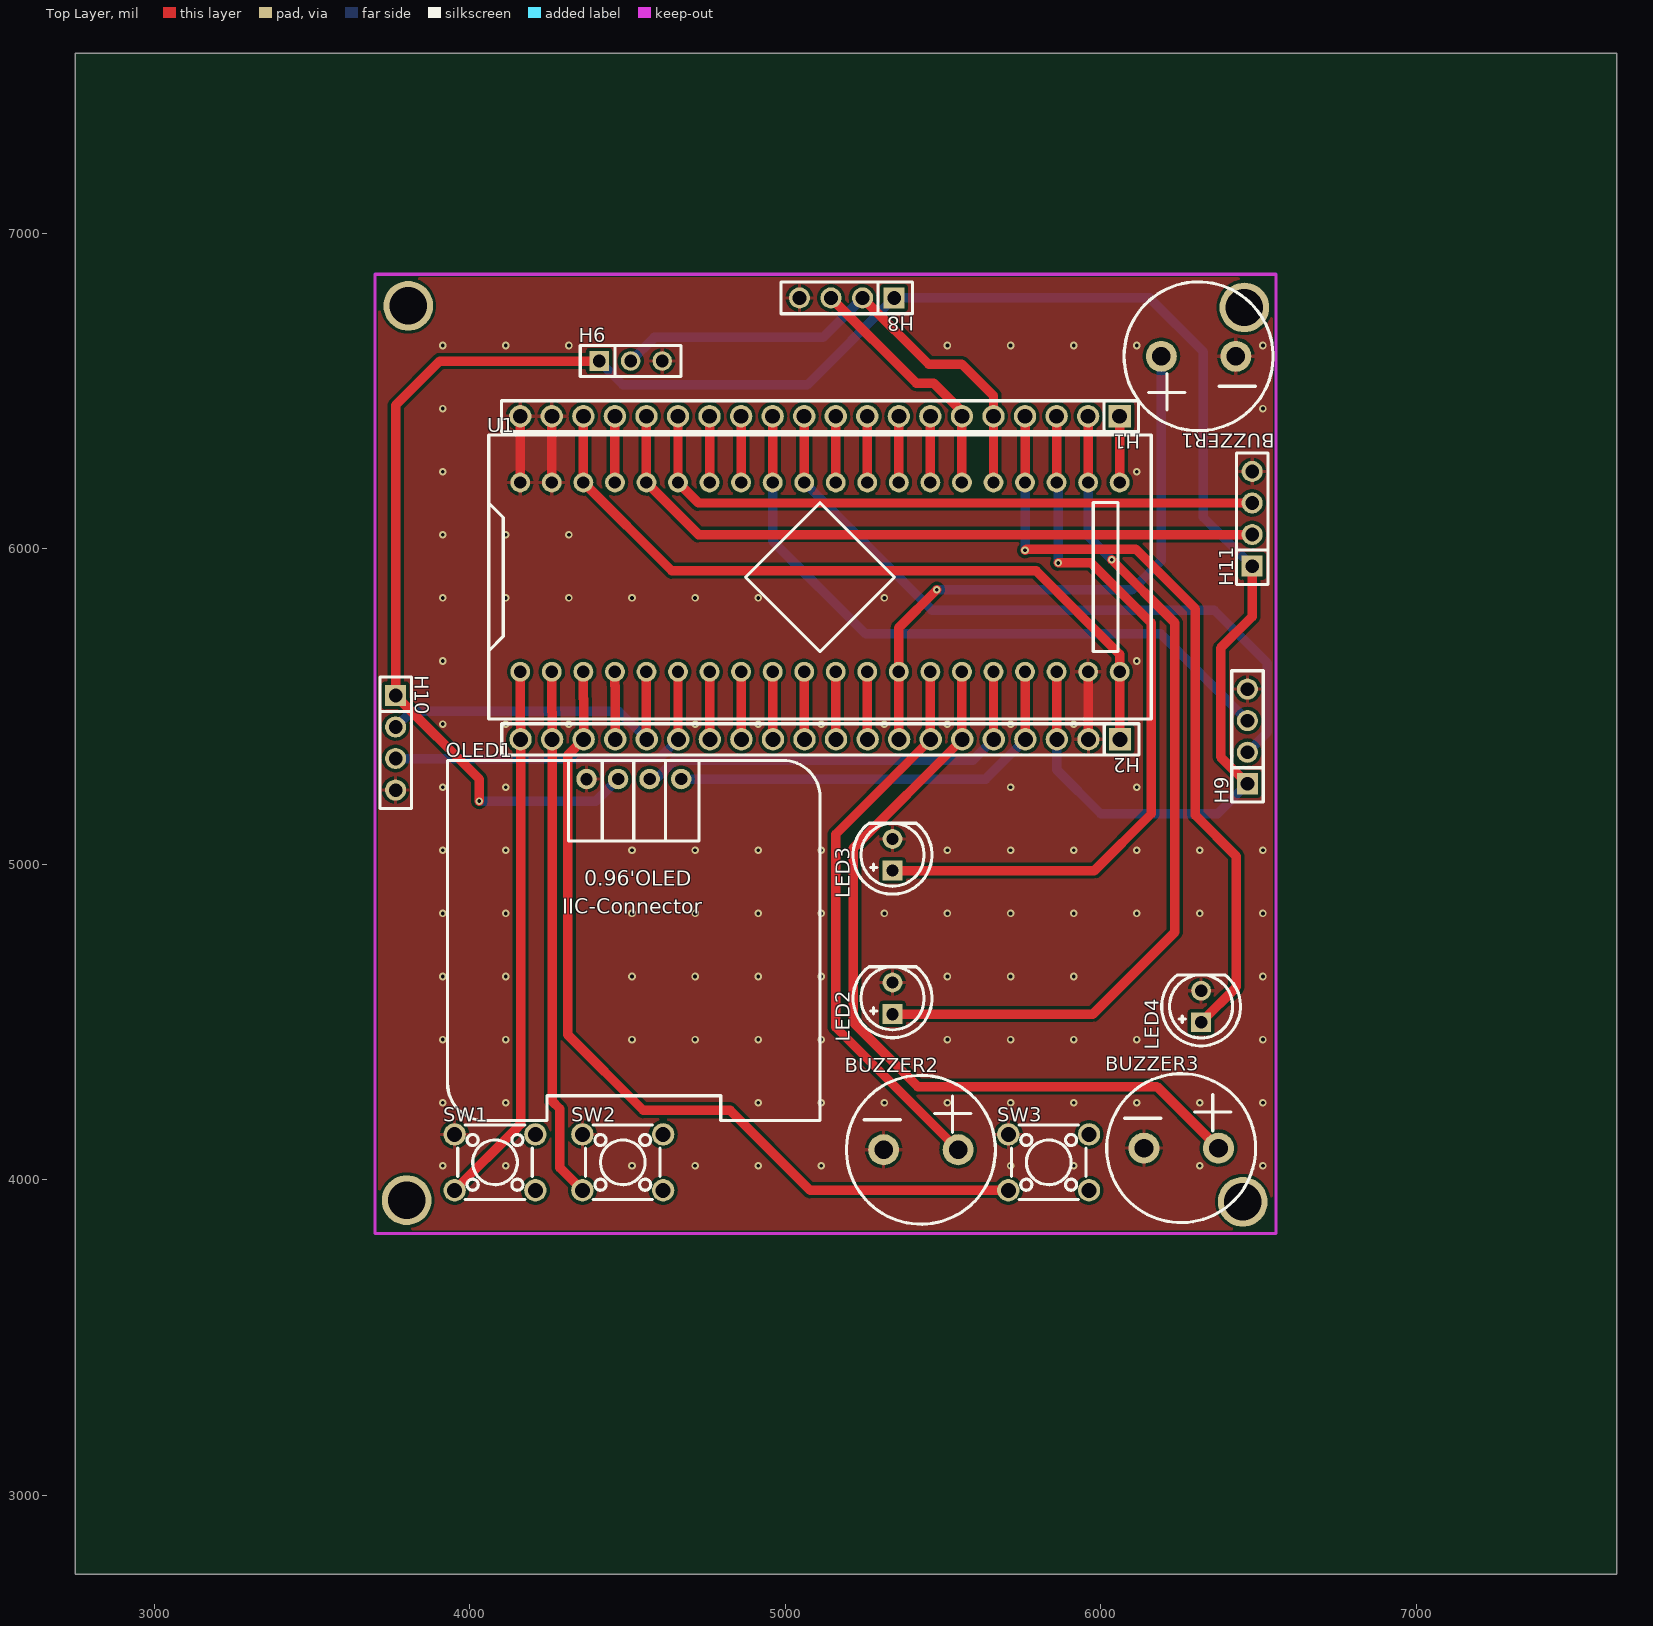
[diagram p0: Top Layer view]
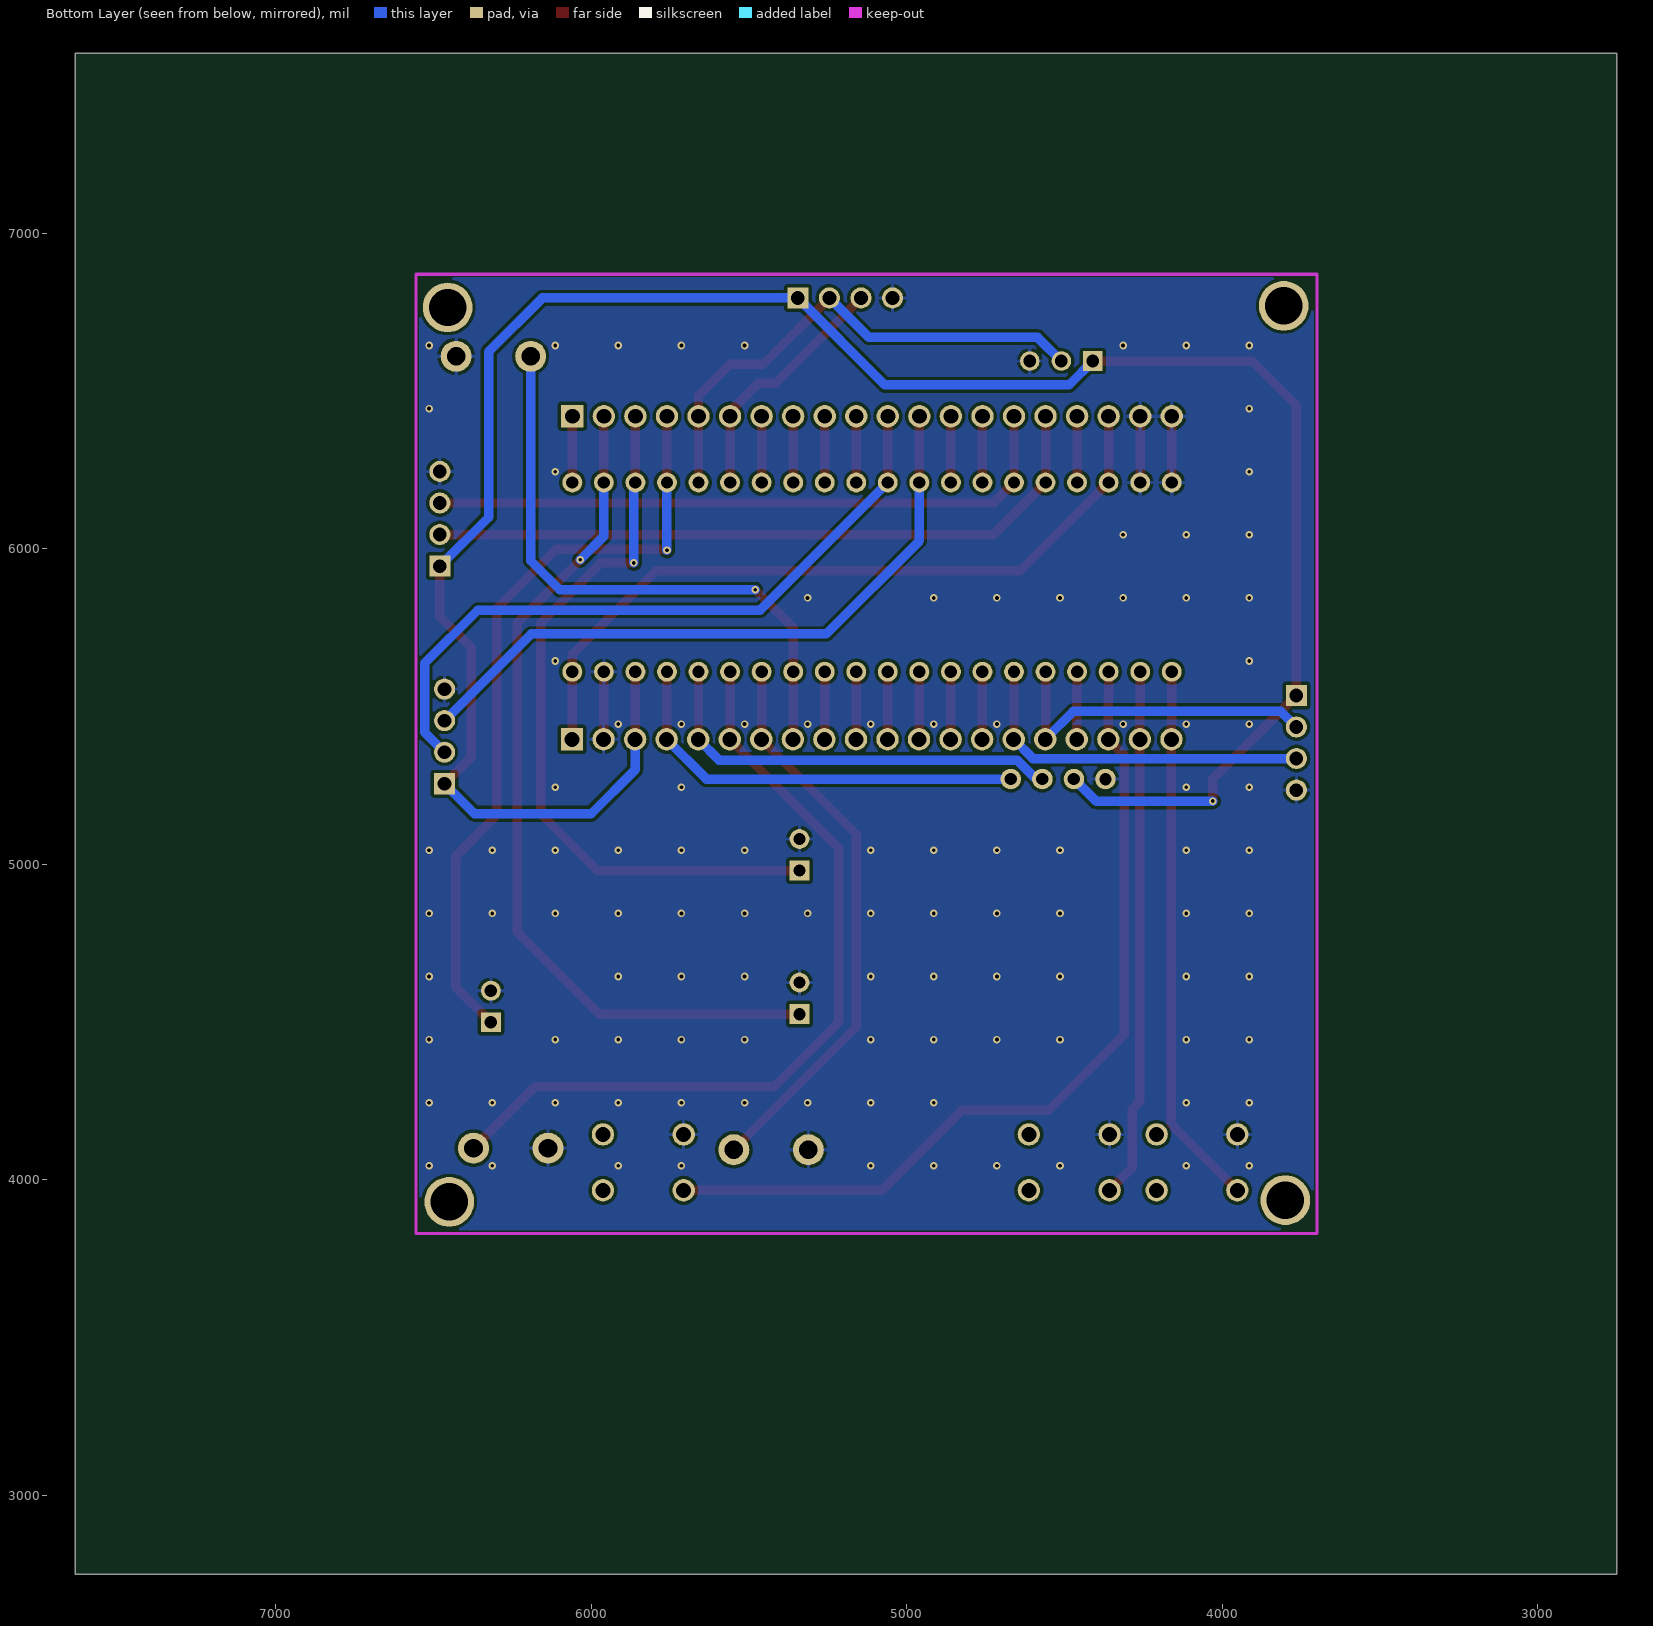
[diagram p1: Bottom Layer view, seen from below]
# Altium PCB MISC51974.pcbdoc
Units mil, origin at the board's own origin, x right, y up, seen from the top; angles counter-clockwise.
Board outline 4885 x 4820 mil, 2 copper layers (Top Layer, Bottom Layer), stack 62.206 mil thick; 18 components, 37 nets, 131 pads, 110 vias.

## Layer stack, top to bottom
Top Solder Mask Layer: solder mask 0.394, Dk 3.3
Top Layer: signal copper 1.379
Dielectric1: surface 59.449, FR4, Dk 4.5
Bottom Layer: signal copper 1.378
Bottom Solder Mask Layer: solder mask 0.394, Dk 3.3

## Board outline
7635,2750 2750,2750 2750,7570 7635,7570

## Design rules (kind name [scope] priority, off if disabled: settings)
BoardOutlineClearance copperThickness2oz_1 [All] p2 off: genericclearance=7.99 ignorepadtopadclearanceinfootprint=FALSE except(0: Arc-SplitContinuation Track-SplitContinuation SMDPad-SplitContinuation THPad-SplitContinuation Via-SplitContinuation Fill-SplitContinuation Region-SplitContinuation Poly-SplitContinuation Text-SplitContinuation Hole-SplitContinuation; 5.98: Arc-CutoutEdge Track-CutoutEdge SMDPad-CutoutEdge THPad-CutoutEdge Via-CutoutEdge Text-CutoutEdge; 6.89: Hole-OutlineEdge Hole-CutoutEdge; 10: Poly-OutlineEdge Poly-CutoutEdge; 11.81: Arc-OutlineEdge Track-OutlineEdge SMDPad-OutlineEdge THPad-OutlineEdge Via-OutlineEdge Fill-OutlineEdge Region-OutlineEdge Text-OutlineEdge Fill-CutoutEdge Region-CutoutEdge)
BoardOutlineClearance Plane_innerPlane_1 [All] p4 off: genericclearance=4.02 ignorepadtopadclearanceinfootprint=FALSE except(0: Arc-SplitContinuation Track-SplitContinuation SMDPad-SplitContinuation THPad-SplitContinuation Via-SplitContinuation Fill-SplitContinuation Region-SplitContinuation Poly-SplitContinuation Text-SplitContinuation Hole-SplitContinuation; 5.98: Arc-CutoutEdge Track-CutoutEdge SMDPad-CutoutEdge THPad-CutoutEdge Via-CutoutEdge Text-CutoutEdge; 6.89: Hole-OutlineEdge Hole-CutoutEdge; 10: Poly-OutlineEdge Poly-CutoutEdge; 11.81: Arc-OutlineEdge Track-OutlineEdge SMDPad-OutlineEdge THPad-OutlineEdge Via-OutlineEdge Fill-OutlineEdge Region-OutlineEdge Text-OutlineEdge Fill-CutoutEdge Region-CutoutEdge)
BoardOutlineClearance Copper_copperRegion_1 [All] p6 off: genericclearance=4.02 ignorepadtopadclearanceinfootprint=FALSE except(0: Arc-SplitContinuation Track-SplitContinuation SMDPad-SplitContinuation THPad-SplitContinuation Via-SplitContinuation Fill-SplitContinuation Region-SplitContinuation Poly-SplitContinuation Text-SplitContinuation Hole-SplitContinuation; 5.98: Arc-CutoutEdge Track-CutoutEdge SMDPad-CutoutEdge THPad-CutoutEdge Via-CutoutEdge Text-CutoutEdge; 6.89: Hole-OutlineEdge Hole-CutoutEdge; 10: Poly-OutlineEdge Poly-CutoutEdge; 11.81: Arc-OutlineEdge Track-OutlineEdge SMDPad-OutlineEdge THPad-OutlineEdge Via-OutlineEdge Fill-OutlineEdge Region-OutlineEdge Text-OutlineEdge Fill-CutoutEdge Region-CutoutEdge)
BoardOutlineClearance copperThickness1oz_1 [All] p8: genericclearance=4.02 ignorepadtopadclearanceinfootprint=FALSE except(0: Arc-SplitContinuation Track-SplitContinuation SMDPad-SplitContinuation THPad-SplitContinuation Via-SplitContinuation Fill-SplitContinuation Region-SplitContinuation Poly-SplitContinuation Text-SplitContinuation Hole-SplitContinuation; 5.98: Arc-CutoutEdge Track-CutoutEdge SMDPad-CutoutEdge THPad-CutoutEdge Via-CutoutEdge Text-CutoutEdge; 6.89: Hole-OutlineEdge Hole-CutoutEdge; 10: Poly-OutlineEdge Poly-CutoutEdge; 11.81: Arc-OutlineEdge Track-OutlineEdge SMDPad-OutlineEdge THPad-OutlineEdge Via-OutlineEdge Fill-OutlineEdge Region-OutlineEdge Text-OutlineEdge Fill-CutoutEdge Region-CutoutEdge)
Clearance copperThickness2oz [All] p1 off: gap=7.99 ignorepadtopadclearanceinfootprint=FALSE except(5.98: SMDPad-Track SMDPad-SMDPad THPad-Track SMDPad-THPad THPad-THPad Track-Via SMDPad-Via THPad-Via Via-Via Fill-SMDPad Region-SMDPad Fill-THPad Region-THPad Fill-Via Region-Via Fill-Fill Fill-Region Region-Region Arc-Track Arc-SMDPad Arc-THPad Arc-Via Fill-Arc Region-Arc Arc-Arc Text-Track SMDPad-Text Text-THPad Text-Via Fill-Text Region-Text Arc-Text Text-Text; 6.89: Hole-Track Hole-SMDPad Hole-THPad Hole-Via Fill-Hole Region-Hole Hole-Arc Hole-Text; 10: Poly-Track Poly-SMDPad Poly-THPad Poly-Via Poly-Fill Poly-Region Poly-Poly Poly-Arc Poly-Text Poly-Hole; 11.81: Fill-Track Region-Track)
Clearance Plane_innerPlane [All] p3 off: gap=4.02 ignorepadtopadclearanceinfootprint=FALSE except(5.98: SMDPad-Track SMDPad-SMDPad THPad-Track SMDPad-THPad THPad-THPad Track-Via SMDPad-Via THPad-Via Via-Via Fill-SMDPad Region-SMDPad Fill-THPad Region-THPad Fill-Via Region-Via Fill-Fill Fill-Region Region-Region Arc-Track Arc-SMDPad Arc-THPad Arc-Via Fill-Arc Region-Arc Arc-Arc Text-Track SMDPad-Text Text-THPad Text-Via Fill-Text Region-Text Arc-Text Text-Text; 6.89: Hole-Track Hole-SMDPad Hole-THPad Hole-Via Fill-Hole Region-Hole Hole-Arc Hole-Text; 10: Poly-Track Poly-SMDPad Poly-THPad Poly-Via Poly-Fill Poly-Region Poly-Poly Poly-Arc Poly-Text Poly-Hole; 11.81: Fill-Track Region-Track)
Clearance Copper_copperRegion [All] p5 off: gap=4.02 ignorepadtopadclearanceinfootprint=FALSE except(5.98: SMDPad-Track SMDPad-SMDPad THPad-Track SMDPad-THPad THPad-THPad Track-Via SMDPad-Via THPad-Via Via-Via Fill-SMDPad Region-SMDPad Fill-THPad Region-THPad Fill-Via Region-Via Fill-Fill Fill-Region Region-Region Arc-Track Arc-SMDPad Arc-THPad Arc-Via Fill-Arc Region-Arc Arc-Arc Text-Track SMDPad-Text Text-THPad Text-Via Fill-Text Region-Text Arc-Text Text-Text; 6.89: Hole-Track Hole-SMDPad Hole-THPad Hole-Via Fill-Hole Region-Hole Hole-Arc Hole-Text; 10: Poly-Track Poly-SMDPad Poly-THPad Poly-Via Poly-Fill Poly-Region Poly-Poly Poly-Arc Poly-Text Poly-Hole; 11.81: Fill-Track Region-Track)
Clearance copperThickness1oz [All] p7: gap=4.02 ignorepadtopadclearanceinfootprint=FALSE except(5.98: SMDPad-Track SMDPad-SMDPad THPad-Track SMDPad-THPad THPad-THPad Track-Via SMDPad-Via THPad-Via Via-Via Fill-SMDPad Region-SMDPad Fill-THPad Region-THPad Fill-Via Region-Via Fill-Fill Fill-Region Region-Region Arc-Track Arc-SMDPad Arc-THPad Arc-Via Fill-Arc Region-Arc Arc-Arc Text-Track SMDPad-Text Text-THPad Text-Via Fill-Text Region-Text Arc-Text Text-Text; 6.89: Hole-Track Hole-SMDPad Hole-THPad Hole-Via Fill-Hole Region-Hole Hole-Arc Hole-Text; 10: Poly-Track Poly-SMDPad Poly-THPad Poly-Via Poly-Fill Poly-Region Poly-Poly Poly-Arc Poly-Text Poly-Hole; 11.81: Fill-Track Region-Track)
DiffPairsRouting differentialPair [All] p1: maxlimit=6 minlimit=6 mostfreqgap=6 toplayer_minwidth=5 toplayer_prefwidth=10 toplayer_maxwidth=100 toplayer_mingap=6 toplayer_prefgap=6 toplayer_maxgap=6 bottomlayer_minwidth=5 bottomlayer_prefwidth=10 bottomlayer_maxwidth=100 bottomlayer_mingap=6 bottomlayer_prefgap=6 bottomlayer_maxgap=6 maxuncoupledlength=10
HoleToHoleClearance otherClearance [All] p1: gap=11.81 allowstackedmicrovias=TRUE
Length netLength [All] p1: minlimit=0 maxlimit=0
PasteMaskExpansion pasteMaskExpansion [All] p1: expansion=0
PlaneConnect innerPlane [All] p1: planeconnectstyle=Relief reliefexpansion=20 reliefentries=4 reliefconductorwidth=10 reliefairgap=10
PolygonConnect copperRegion [All] p1: connectstyle=Relief reliefconductorwidth=10 reliefentries=4 polygonreliefangle="90 Angle" airgapwidth=10 via.connectstyle=Relief via.reliefconductorwidth=10 via.reliefentries=4 via.polygonreliefangle="90 Angle" via.airgapwidth=10
RoutingVias viaSize [All] p1: holewidth=12.01 width=24.02 viastyle="Through Hole" minholewidth=11.81 minwidth=19.68 maxholewidth=248.03 maxwidth=393.7
SolderMaskExpansion solderMaskExpansion [IsVia] p1: expansion=-1000 istentingtop=TRUE
SolderMaskExpansion solderMaskExpansion [All] p2: expansion=2.01 istentingtop=FALSE
Width copperThickness2oz_2 [All] p1 off: maxlimit=100 minlimit=8 preferedwidth=10
Width copperThickness1oz_2 [All] p2: maxlimit=100 minlimit=5 preferedwidth=30

## Components (designator, comment, footprint, x,y, rotation, side; value= is the part's Value field where it differs from the comment)
BUZZER1 "buzzer" BUZ-TH_BD12.0-P6.00-D0.9-RD 6310,6610 r180 top
BUZZER2 "buzzer" BUZ-TH_BD12.0-P6.00-D0.9-RD 5430,4095 r0 top
BUZZER3 "buzzer" BUZ-TH_BD12.0-P6.00-D0.9-RD 6255,4100 r0 top
H1 "" HDR-TH_20P-P2.54-V-F 5110,6420 r180 top
H2 "" HDR-TH_20P-P2.54-V-F 5110.96,5395.9 r180 top
H6 "" HDR-TH_3P-P2.54-V-F 4510,6595 r0 top
H8 "" HDR-TH_4P-P2.54-V-F 5195,6795 r180 top
H9 "" HDR-TH_4P-P2.54-V-F 6465,5405 r90 top
H10 "" HDR-TH_4P-P2.54-V-F 3765,5385 r270 top
H11 "" HDR-TH_4P-P2.54-V-F 6480,6095 r90 top
LED2 "" LED-TH_5mm 5340,4575 r90 top
LED3 "" LED-TH_5mm 5340,5030 r90 top
LED4 "" LED-TH_5mm 6318.09,4549.15 r90 top
OLED1 "" 0.96OLED_4P 4520,5270 r0 top
SW1 "" SW-TH_4P-L6.0-W6.0-P4.50-LS6.5 4080,4055 r0 top
SW2 "" SW-TH_4P-L6.0-W6.0-P4.50-LS6.5 4485,4055 r0 top
SW3 "" SW-TH_4P-L6.0-W6.0-P4.50-LS6.5 5835,4055 r0 top
U1 "STM32F103C8T6-Card" CONN-TH_L53.3-W22.9_STM32F103C8T6-CARD 5110,5910 r0 top

## Footprints (in the part's own frame and the unit in brackets; to place one, negate y for a bottom-side part, rotate by r counter-clockwise, add the part's x,y. Pads: shape width x height; smd on the part's side, far side on the other; paste and mask are expansions set on the pad)
0.96OLED_4P [mm]
  round 1.65 hole 1 copper offset 0,0: 1(-3.81,-0.001) 2(-1.27,0.002) 3(1.27,0.002) 4(3.81,0.002)
  silkscreen extent -15,-27.5 15,1.5
BUZ-TH_BD12.0-P6.00-D0.9-RD [mm]
  round 2.5 hole 1.5 paste+0 mask+0.05: 1(-3,0) 2(3,0)
  silkscreen extent -5.99,-5.99 5.99,5.99
CONN-TH_L53.3-W22.9_STM32F103C8T6-CARD [mm]
  round 1.6 hole 1: 1(-24.13,-7.62) 2(-21.59,-7.62) 3(-19.05,-7.62) 4(-16.51,-7.62) 5(-13.97,-7.62) 6(-11.43,-7.62) 7(-8.89,-7.62) 8(-6.35,-7.62) 9(-3.81,-7.62) 10(-1.27,-7.62) 11(1.27,-7.62) 12(3.81,-7.62) 13(6.35,-7.62) 14(8.89,-7.62) 15(11.43,-7.62) 16(13.97,-7.62) 17(16.51,-7.62) 18(19.05,-7.62) 19(21.59,-7.62) 20(24.13,-7.62) 21(24.13,7.62) 22(21.59,7.62) 23(19.05,7.62) 24(16.51,7.62) 25(13.97,7.62) 26(11.43,7.62) 27(8.89,7.62) 28(6.35,7.62) 29(3.81,7.62) 30(1.27,7.62) 31(-1.27,7.62) 32(-3.81,7.62) 33(-6.35,7.62) 34(-8.89,7.62) 35(-11.43,7.62) 36(-13.97,7.62) 37(-16.51,7.62) 38(-19.05,7.62) 39(-21.59,7.62) 40(-24.13,7.62)
  silkscreen extent -26.67,-11.43 26.67,11.43
HDR-TH_3P-P2.54-V-F [mil]
  rect 62x62 hole 40.16: 1(-100,0)
  round 62 hole 40.16: 2(0,0) 3(100,0)
  silkscreen extent -160,-49 160,49
HDR-TH_4P-P2.54-V-F [mm]
  rect 1.7x1.7 hole 1.1: 1(-3.81,0)
  round 1.7 hole 1.1: 2(-1.27,0) 3(1.27,0) 4(3.81,0)
  silkscreen extent -5.29,-1.27 5.29,1.27
HDR-TH_20P-P2.54-V-F [mm]
  rect 1.8x1.8 hole 1.2: 1(-24.13,0)
  round 1.8 hole 1.2: 2(-21.59,0) 3(-19.05,0) 4(-16.51,0) 5(-13.97,0) 6(-11.43,0) 7(-8.89,0) 8(-6.35,0) 9(-3.81,0) 10(-1.27,0) 11(1.27,0) 12(3.81,0) 13(6.35,0) 14(8.89,0) 15(11.43,0) 16(13.97,0) 17(16.51,0) 18(19.05,0) 19(21.59,0) 20(24.13,0)
  silkscreen extent -25.65,-1.25 25.65,1.25
LED-TH_5mm [mm]
  rect 1.6x1.6 hole 1 paste+0 mask+0.051: 1(-1.27,0)
  round 1.6 hole 1 paste+0 mask+0.051: 2(1.27,0)
  silkscreen extent -3.17,-3.17 2.54,3.17
SW-TH_4P-L6.0-W6.0-P4.50-LS6.5 [mm]
  round 1.8 hole 1.2: 1(-3.25,2.25) 2(3.25,2.25) 3(-3.25,-2.25) 4(3.25,-2.25)
  silkscreen extent -3,-3 3,3

## Free pads (board coordinates)
  round 157.48 hole 118.11: 1(3800,3935) 1(3805,6770) 1(6450,3930) 1(6455,6765)

## Via types
v1: diameter 24.02, hole 12, Top Layer to Bottom Layer, 110 vias

## Nets (pads, with @x,y where several pads share a name; then routed paths per layer and width w, separated by ;. In a path a pad name is that pad's centre, name@x,y a point inside that pad or via, vN(x,y) a via of type N, cw(c..) or ccw(c..) an arc to the next point about the centre after c; other vN are vias at no path point)
+5V: H2.3 H6.1 H8.1 H9.1 H10.1 H11.1 OLED1.2 U1.18 | length 7190.3
  Top Layer w30: v1(4030,5200) 4030,5270 H10.1 3765,6455 3905,6595 H6.1 ; U1.18 5860,5396.86 H2.3 ; H9.1 6380,5340 6380,5685 6480,5785 H11.1
  Bottom Layer w30: v1(4030,5200) 4399.95,5200 OLED1.2@4470,5270.05 ; H6.1 4485,6520 5070,6520 H8.1 6155,6795 6325,6625 6325,6100 H11.1 ; H2.3 5860.96,5299.04 6000,5160 6370,5160 H9.1
GND: BUZZER1.1 BUZZER2.1 BUZZER3.1 H1.19 H1.20 H2.2 H6.3 H8.4 H9.4 H10.4 H11.4 LED2.2 LED3.2 LED4.2 OLED1.1 SW1.1 SW2.1 SW3.1 U1.19 U1.39 U1.40 | length 634.5
  Top Layer w30: U1.40 H1.20 ; U1.39 H1.19 ; U1.19 5960,5396.86 H2.2
  other v1: 3914.1,4044.1 4114.1,4044.1 4514.1,4044.1 4714.1,4044.1 4914.1,4044.1 5114.1,4044.1 5714.1,4044.1 5914.1,4044.1 6314.1,4044.1 6514.1,4044.1 3914.1,4244.1 4114.1,4244.1 4914.1,4244.1 5114.1,4244.1 5314.1,4244.1 5514.1,4244.1 5714.1,4244.1 5914.1,4244.1 6114.1,4244.1 6314.1,4244.1 6514.1,4244.1 3914.1,4444.1 4114.1,4444.1 4514.1,4444.1 4714.1,4444.1 4914.1,4444.1 5114.1,4444.1 5514.1,4444.1 5714.1,4444.1 5914.1,4444.1 6114.1,4444.1 6514.1,4444.1 3914.1,4644.1 4114.1,4644.1 4514.1,4644.1 4714.1,4644.1 4914.1,4644.1 5114.1,4644.1 5514.1,4644.1 5714.1,4644.1 5914.1,4644.1 6514.1,4644.1 3914.1,4844.1 4114.1,4844.1 4514.1,4844.1 4714.1,4844.1 4914.1,4844.1 5114.1,4844.1 5314.1,4844.1 5514.1,4844.1 5714.1,4844.1 5914.1,4844.1 6114.1,4844.1 6314.1,4844.1 6514.1,4844.1 3914.1,5044.1 4114.1,5044.1 4514.1,5044.1 4714.1,5044.1 4914.1,5044.1 5114.1,5044.1 5514.1,5044.1 5714.1,5044.1 5914.1,5044.1 6114.1,5044.1 6314.1,5044.1 6514.1,5044.1 3914.1,5244.1 4114.1,5244.1 5714.1,5244.1 6114.1,5244.1 3914.1,5444.1 4114.1,5444.1 4314.1,5444.1 4714.1,5444.1 4914.1,5444.1 5114.1,5444.1 5314.1,5444.1 5514.1,5444.1 5714.1,5444.1 5914.1,5444.1 3914.1,5644.1 6114.1,5644.1 3914.1,5844.1 4114.1,5844.1 4314.1,5844.1 4514.1,5844.1 4714.1,5844.1 4914.1,5844.1 5314.1,5844.1 3914.1,6044.1 4114.1,6044.1 4314.1,6044.1 3914.1,6244.1 6114.1,6244.1 3914.1,6444.1 6514.1,6444.1 3914.1,6644.1 4114.1,6644.1 4314.1,6644.1 5514.1,6644.1 5714.1,6644.1 5914.1,6644.1 6114.1,6644.1 6514.1,6644.1
NRST: H1.17 U1.37 | length 210
  Top Layer w30: U1.37 H1.17
PA0: H1.5 H6.2 H8.2 U1.25 | length 1636.2
  Top Layer w30: H8.2 5455,6585 5560,6585 5660,6485 H1.5 U1.25
  Bottom Layer w30: H6.2 4585,6670 5120,6670 H8.2
PA1: H1.6 H8.3 U1.26 | length 789.1
  Top Layer w30: H8.3 5415,6525 5470,6525 5560,6435 H1.6 U1.26
PA2: H1.7 U1.27 | length 210
  Top Layer w30: U1.27 H1.7
PA3: H1.8 U1.28 | length 210
  Top Layer w30: U1.28 H1.8
PA4: H1.9 U1.29 | length 210
  Top Layer w30: U1.29 H1.9
PA5: H1.10 U1.30 | length 210
  Top Layer w30: U1.30 H1.10
PA6: H1.11 H9.2 U1.31 | length 2223.6
  Top Layer w30: U1.31 H1.11
  Bottom Layer w30: U1.31 5465,5805 6360,5805 6528.19,5636.81 6528.19,5418.19 H9.2
PA7: H1.12 H9.3 U1.32 | length 2136.1
  Top Layer w30: U1.32 H1.12
  Bottom Layer w30: U1.32 4960,6025 5255,5730 6190,5730 H9.3
PA8: H2.16 H10.2 U1.5 | length 1068.1
  Top Layer w30: U1.5 4560,5396.86 H2.16
  Bottom Layer w30: H10.2 3815,5485 4471.86,5485 H2.16
PA9: H2.15 H10.3 U1.6 | length 1135.7
  Top Layer w30: U1.6 4660,5396.86 H2.15
  Bottom Layer w30: H10.3 4600.06,5335 H2.15
PA10: H2.14 U1.7 | length 214.5
  Top Layer w30: U1.7 4760,5396.86 H2.14
PA11: H2.13 U1.8 | length 214.5
  Top Layer w30: U1.8 4860,5396.86 H2.13
PA12: H2.12 U1.9 | length 214.5
  Top Layer w30: U1.9 4960,5396.86 H2.12
PA15: H2.11 U1.10 | length 214.5
  Top Layer w30: U1.10 5060,5396.86 H2.11
PB0: H1.13 U1.33 | length 210
  Top Layer w30: U1.33 H1.13
PB1: H1.14 U1.34 | length 210
  Top Layer w30: U1.34 H1.14
PB3: H2.10 U1.11 | length 214.5
  Top Layer w30: U1.11 5160,5396.86 H2.10
PB4: H2.9 U1.12 | length 214.5
  Top Layer w30: U1.12 5260,5396.86 H2.9
PB5: BUZZER1.2 H2.8 U1.13 | length 1922.3
  Top Layer w30: H2.8 5360,5396.86 U1.13 5360,5750 v1(5480,5870)
  Bottom Layer w30: v1(5480,5870) 6100,5870 6191.89,5961.89 BUZZER1.2
PB6: BUZZER2.2 H2.7 U1.14 | length 1800.8
  Top Layer w30: U1.14 5460,5396.86 H2.7 5160,5094.94 5160,4483.11 BUZZER2.2
PB7: BUZZER3.2 H2.6 U1.15 | length 2577.5
  Top Layer w30: U1.15 5560,5396.86 H2.6 5215,5049.94 5215,4500 5420,4295 6178.11,4295 BUZZER3.2
PB8: H2.5 OLED1.3 U1.16 | length 1357.6
  Top Layer w30: U1.16 5660,5396.86 H2.5
  Bottom Layer w30: OLED1.3@4570,5270.05 4590.05,5270.05 4650,5330 5595.06,5330 H2.5
PB9: H2.4 OLED1.4 U1.17 | length 1357.6
  Top Layer w30: U1.17 5760,5396.86 H2.4
  Bottom Layer w30: OLED1.4@4670,5270.05 5635.11,5270.05 H2.4
PB10: H1.15 H11.3 U1.35 | length 2056.9
  Top Layer w30: H1.15 U1.35 4725,6145 H11.3
PB11: H1.16 H11.2 U1.36 | length 2198.3
  Top Layer w30: H1.16 U1.36 4725,6045 H11.2
PB12: H2.20 SW1.3 U1.1 | length 1730.5
  Top Layer w30: SW1.3 4151.53,4165.9 4151.53,4166.95 4160.96,4176.38 H2.20 4160.96,5441.33 4160,5442.29 U1.1
PB13: H2.19 SW2.3 U1.2 | length 1683.8
  Top Layer w30: U1.2 4260,5483.71 4260.96,5482.75 H2.19 4260.96,4249.04 4285,4225 4285,4038.47 SW2.3
PB14: H2.18 SW3.3 U1.3 | length 2773
  Top Layer w30: U1.3 4360,5525.13 4360.96,5524.17 H2.18 4310,5344.94 4310,4460 4550,4220 4825,4220 5078.58,3966.42 SW3.3
PB15: H2.17 U1.4 | length 214.5
  Top Layer w30: U1.4 4460,5566.55 4460.96,5565.59 H2.17
PC13: H1.2 LED2.1 U1.22 | length 2751.6
  Top Layer w30: LED2.1 5975,4525 6235,4785 6235,5765 v1(6035,5965) ; U1.22 H1.2
  Bottom Layer w30: U1.22 5960,6040 v1(6035,5965)
PC14: H1.3 LED3.1 U1.23 | length 2340.3
  Top Layer w30: LED3.1 5980,4980 6160,5160 6160,5765 5970,5955 v1(5865,5955) ; U1.23 H1.3
  Bottom Layer w30: U1.23 5865,6205 v1(5865,5955)
PC15: H1.4 LED4.1 U1.24 | length 2456
  Top Layer w30: v1(5760,5995) 5764.02,5999.02 6110.98,5999.02 6300,5810 6300,5155 6430,5025 6430,4611.06 LED4.1 ; U1.24 H1.4
  Bottom Layer w30: v1(5760,5995) U1.24
VBAT: H1.1 U1.21 | length 210
  Top Layer w30: U1.21 H1.1
VCC: H1.18 H2.1 U1.20 U1.38 | length 2405.2
  Top Layer w30: H1.18 U1.38 4640,5930 5795,5930 6060,5665 U1.20 6060,5396.86 H2.1
pads on no net: SW1.2 SW1.4 SW2.2 SW2.4 SW3.2 SW3.4

## Polygon pours and split planes (outlines as drawn)
GND on Bottom Layer (solid, remove dead copper, pour order 2): 3100,7165 3100,3000 7275,3000 7275,7165
GND on Top Layer (solid, remove dead copper, pour order 0): 3000,7320 3000,3250 7385,3250 7385,7320

## Keep-outs
Board Outline Layer:
  lines w10: 3700,3830 3700,6870 6555,6870 6555,3830 3700,3830